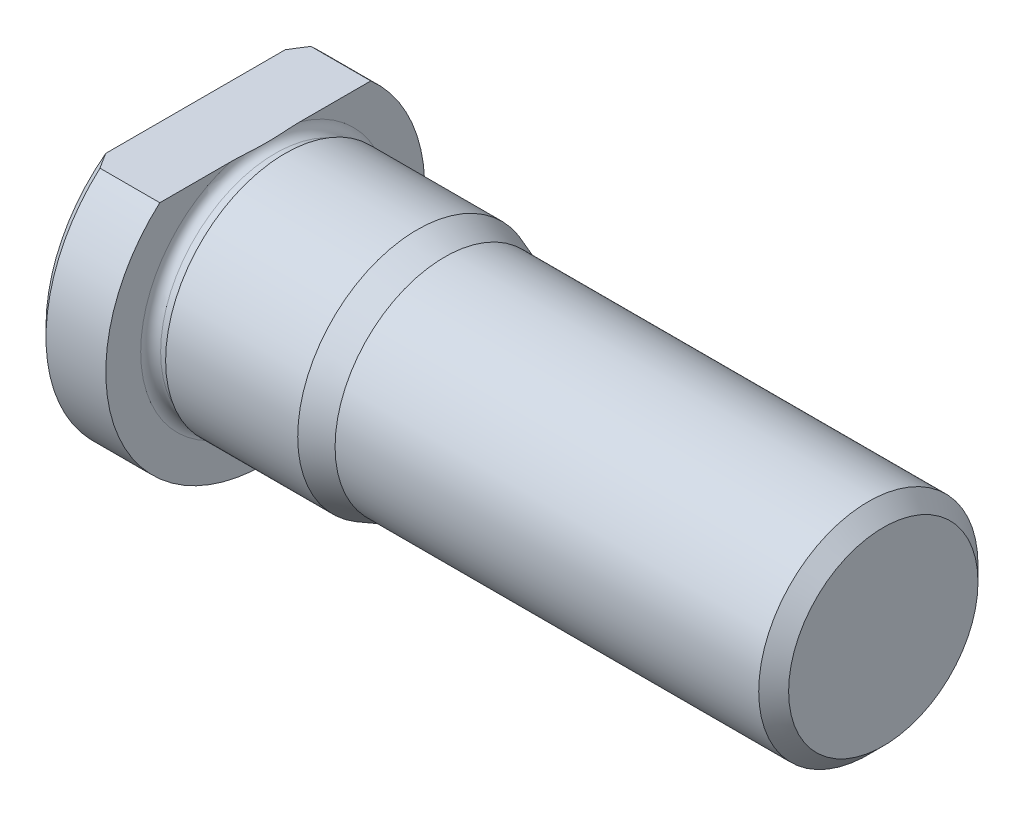
from build123d import *

# Parameters (mm, degrees)
CHAMFER_1_SIZE      = 1
FILLET_1_R          = 1
CHAMFER_3_SIZE      = 1.5
CUT_EXTRUDE_START   = 8
CUT_EXTRUDE_5_DEPTH = 8


with BuildPart() as part:
    # 草图1 → 旋转1 (revolve)
    with BuildSketch(Plane.XY, mode=Mode.PRIVATE) as revolve_1_sk:
        Polygon((0, 0), (0, 16), (7, 16), (7, 11.5), (9, 11.5), (9, 12), (22.252522581, 12), (25, 11), (69, 11), (69, 0), align=None)
    revolve(revolve_1_sk.sketch.rotate(Axis((-47.69348659, 0, 0), (1, 0, 0)), 90), axis=Axis((-47.69348659, 0, 0), (1, 0, 0)))

    # 倒角1
    chamfer_1_edges = [part.edges().sort_by_distance(p)[0] for p in [
        (0, 0, -16),
    ]]
    chamfer(chamfer_1_edges, length=CHAMFER_1_SIZE)

    # 圆角1
    fillet_1_edges = [part.edges().sort_by_distance(p)[0] for p in [
        (7, 0, -11.5),
    ]]
    fillet(fillet_1_edges, radius=FILLET_1_R)

    # 倒角3
    chamfer_3_edges = [part.edges().sort_by_distance(p)[0] for p in [
        (69, 0, -11),
    ]]
    chamfer(chamfer_3_edges, length=CHAMFER_3_SIZE)

    # 草图2 → 切除-拉伸5 (cut)
    with BuildSketch(Plane(origin=(0, 0, 0), x_dir=(0, 0, -1), z_dir=(1, 0, 0)).offset(CUT_EXTRUDE_START)):
        with BuildLine():
            Line((-10.583005244, 12), (10.583005244, 12))
            ThreePointArc((10.583005244, 12), (0, 16), (-10.583005244, 12))
        make_face()
    extrude(amount=-CUT_EXTRUDE_5_DEPTH, mode=Mode.SUBTRACT)


solid = part.part
